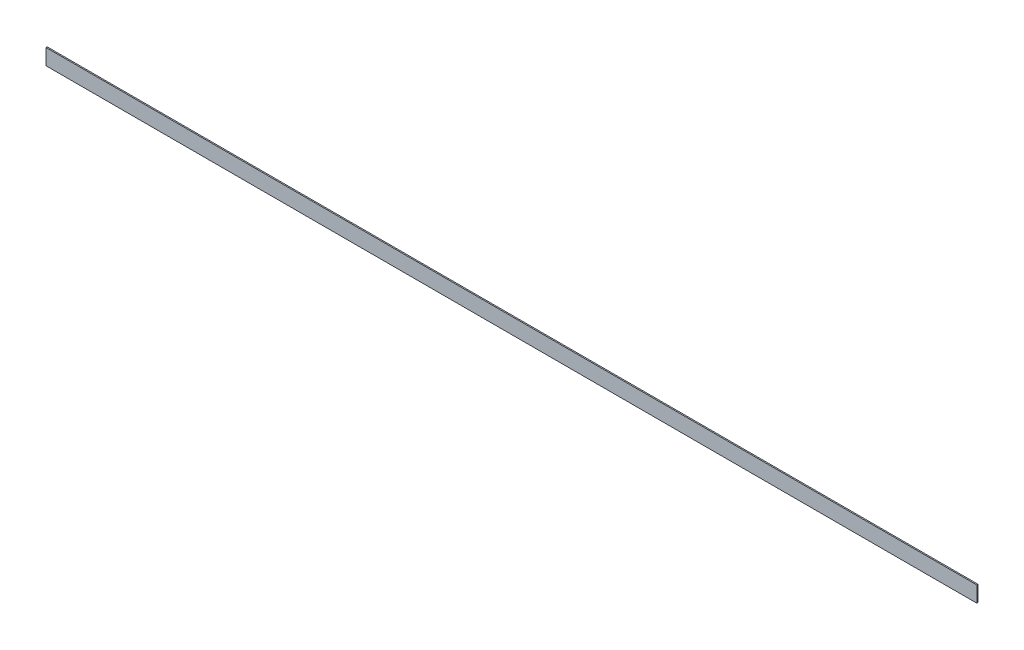
SolidWorks part; units mm, degrees
ref_plane "Front Plane" through (0, 0, 0) normal (0, 0, 1) x (1, 0, 0)
ref_plane "Top Plane" through (0, 0, 0) normal (0, 1, 0) x (1, 0, 0)
ref_plane "Right Plane" through (0, 0, 0) normal (1, 0, 0) x (0, 0, -1)
other "Configuration Table"
sketch "Sketch1" plane through (0, 0, 0) normal (0, 0, 1) x (1, 0, 0)
  line L1 (0, 0) -> (2350, 0)
  line L2 (0, 0) -> (0, -40)
  line L3 (0, -40) -> (2350, -40)
  line L4 (2350, 0) -> (2350, -40)
  dimension "D1" = 2350
  dimension "D2" = 40
extrude "Boss-Extrude1" add sketch "Sketch1" along normal blind 3
